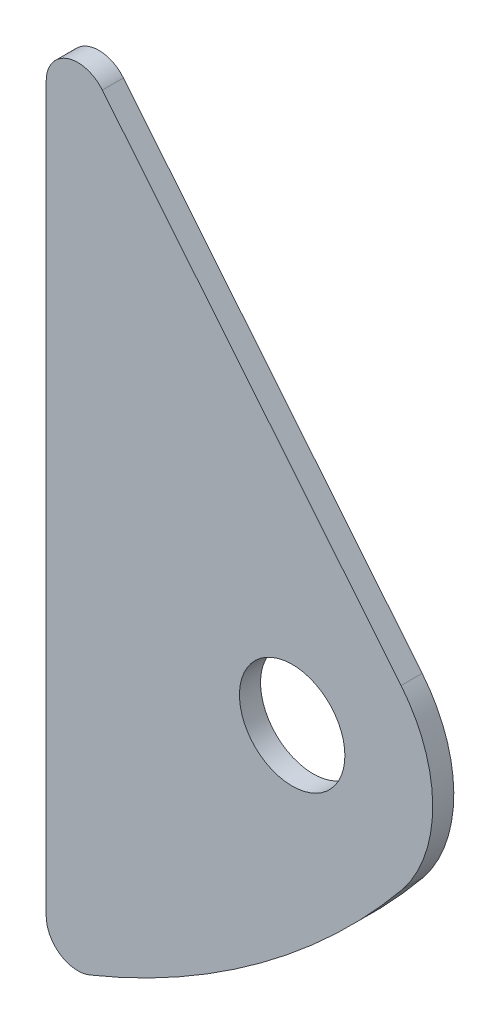
SolidWorks part; units mm, degrees
ref_plane "Front Plane" through (0, 0, 0) normal (0, 0, 1) x (1, 0, 0)
ref_plane "Top Plane" through (0, 0, 0) normal (0, 1, 0) x (1, 0, 0)
ref_plane "Right Plane" through (0, 0, 0) normal (1, 0, 0) x (0, 0, -1)
sketch "Sketch1" plane through (0, 0, 0) normal (0, 0, 1) x (1, 0, 0)
  line L0 (0, 64.77) -> (0, -77.4361) construction
  line L1 (-58.7987, 0) -> (88.8769, 0) construction
  line L2 (-140, 247.6835) -> (-140, -164.0687)
  line L3 (-285, 263.6793) -> (-285, 95.2706) construction
  line L4 (-301.4769, 236) -> (-179.9668, 236) construction
  line L5 (61.9956, 50.5623) -> (-108.051, 259.06)
  circle A0 centre (0, 0) radius 30
  arc A1 (63.0889, -49.1914) -> (61.9956, 50.5623) centre (0, 0) ccw
  arc A2 (-115.2083, -180.7383) -> (63.0889, -49.1914) centre (-285, 236) ccw
  arc A3 (-140, 247.6835) -> (-108.051, 259.06) centre (-122, 247.6835) cw
  arc A4 (-140, -164.0687) -> (-115.2083, -180.7383) centre (-122, -164.0687) ccw
  dimension "D1" = 160
  dimension "D2" = 60
  dimension "D6" = 900
  dimension "D8" = 18
  dimension "D9" = 18
  dimension "D3" = 140
  dimension "D4" = 236
  dimension "D5" = 285
  dimension "D7" = 39.2
extrude "Boss-Extrude1" add sketch "Sketch1" along normal blind 12
